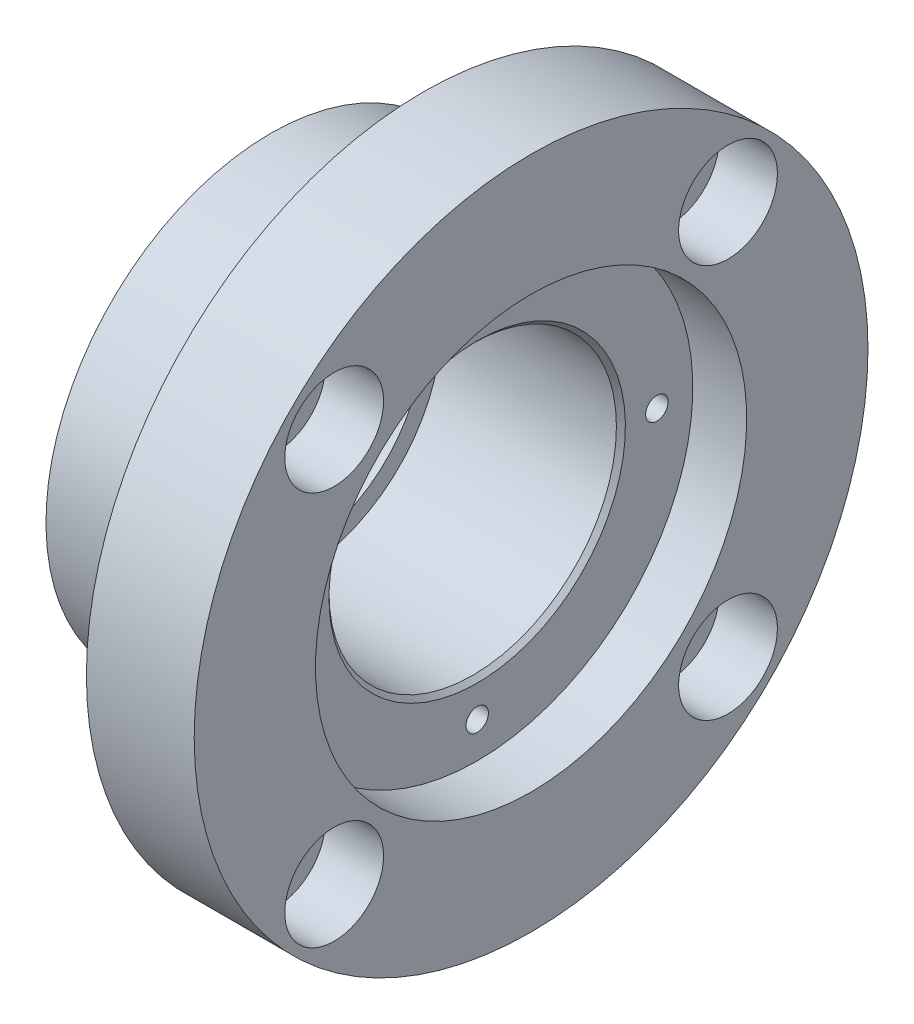
SolidWorks part; units mm, degrees
ref_plane "Front Plane" through (0, 0, 0) normal (0, 0, 1) x (1, 0, 0)
ref_plane "Top Plane" through (0, 0, 0) normal (0, 1, 0) x (1, 0, 0)
ref_plane "Right Plane" through (0, 0, 0) normal (1, 0, 0) x (0, 0, -1)
sketch "Sketch1" plane through (0, 0, 0) normal (0, 0, 1) x (1, 0, 0)
  line L0 (0, 0) -> (-29, 0) construction
  line L1 (0, 24) -> (-6, 24)
  line L2 (-6, 24) -> (-6, 16)
  line L3 (-6, 16) -> (-26, 16)
  line L4 (-26, 16) -> (-26, 14)
  line L5 (-26, 14) -> (-29, 14)
  line L6 (-29, 14) -> (-29, 25)
  line L7 (-29, 25) -> (-12, 25)
  line L8 (-12, 25) -> (-12, 37.5)
  line L9 (-12, 37.5) -> (0, 37.5)
  line L10 (0, 37.5) -> (0, 24)
  line L11 (-17, 16) -> (-17, 0) construction
  line L12 (-8, 16) -> (-8, 0) construction
revolve "Revolve1" add sketch "Sketch1" angle 360 about L0
hole_wizard "CBORE Socket Head Cap Screw1" positions "Sketch3" profile "Sketch2" counterbore size "M6" standard "JIS" end condition up to next
sketch "Sketch3" plane through (0, 0, 0) normal (1, 0, 0) x (0, 0, -1)
  line L2 (0, 0) -> (21.9203, 21.9203) construction
  line L3 (0, 0) -> (21.9203, -21.9203) construction
  circle A0 centre (0, 0) radius 31 construction
  point P0 (-21.9203, 21.9203)
  point P2 (21.9203, 21.9203)
  point P4 (21.9203, -21.9203)
  point P6 (-21.9203, -21.9203)
  dimension "P.C.D." = 62
sketch "Sketch2" plane through (0, 21.9203, 21.9203) normal (0, 1, 0) x (0, 0, -1)
  line L0 (0, 0) -> (0, 12)
  line L1 (0, 12) -> (3.3, 12)
  line L3 (3.3, 12) -> (3.3, 6.5)
  line L4 (3.3, 6.5) -> (5.5, 6.5)
  line L5 (5.5, 6.5) -> (5.5, 0)
  line L7 (5.5, 0) -> (0, 0)
  line L11 (0, 0) -> (0, 12) construction
  dimension "D2_s" = 6.6
  dimension "Thru Hole Depth" = 12
  dimension "D1_s" = 11
  dimension "H1" = 6.5
hole_wizard "Tapped Hole1" positions "Sketch5" profile "Sketch4" tap size "M3x0.5" standard "JIS"
sketch "Sketch5" plane through (-6, 0, 0) normal (1, 0, 0) x (0, 0, -1)
  circle A0 centre (0, 0) radius 20 construction
  point P0 (0, 20)
  point P2 (-20, 0)
  point P4 (0, -20)
  point P6 (20, 0)
  dimension "P.C.D._s" = 40
sketch "Sketch4" plane through (-6, 20, 0) normal (0, 1, 0) x (0, 0, -1)
  line L0 (0, 0) -> (0, 9.2511)
  line L1 (0, 9.2511) -> (1.25, 8.5)
  line L2 (1.25, 8.5) -> (1.25, 0)
  line L5 (1.25, 0) -> (0, 0)
  line L10 (0, 9.2511) -> (-1.25, 8.5) construction
  line L11 (0, 0) -> (0, 9.2511) construction
  dimension "Tap Drill Dia." = 2.5
  dimension "Tap Drill Depth" = 8.5
  dimension "Drill Angle" = 118
cosmetic thread "Hole Thread1"
cosmetic thread "Hole Thread2"
cosmetic thread "Hole Thread3"
cosmetic thread "Hole Thread4"
chamfer "Chamfer1" distance 0.5 angle 45 1 edges at (-6, 16, 0)
equation "\"Bx2@Sketch1\" = \"B@Sketch1\" * 2"
